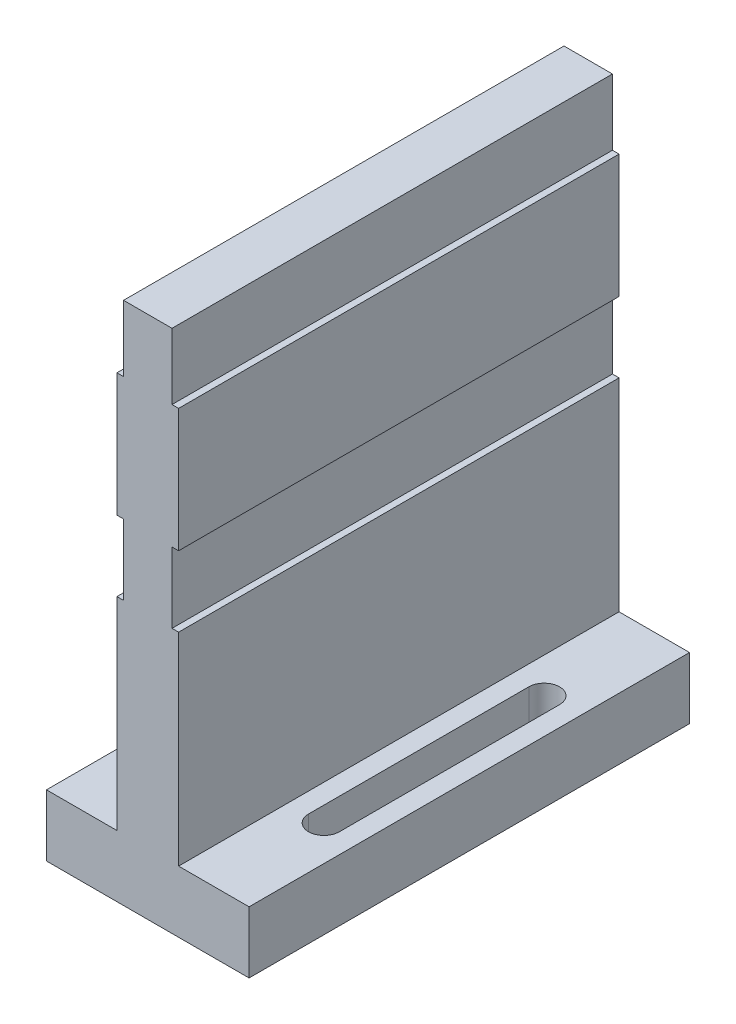
from build123d import *

# Parameters (mm, degrees)
EXTRUDE_1_DEPTH     = 50
CUT_EXTRUDE_1_REACH = 120.55
SKETCH_3_W          = 100
SKETCH_3_H          = 15
SKETCH_3_H_2        = 16
CUT_EXTRUDE_2_DEPTH = 1.5


with BuildPart() as part:
    # 草图1 → 凸台-拉伸1 (new, symmetric)
    with BuildSketch(Plane.XY):
        Polygon((0, 0), (23, 0), (23, 14), (7, 14), (7, 119), (-7, 119), (-7, 14), (-23, 14), (-23, 0), align=None)
    extrude(amount=EXTRUDE_1_DEPTH, both=True)

    # 草图2 → 切除-拉伸1 (cut, up to next)
    with BuildSketch(Plane(origin=(0, 14, 0), x_dir=(1, 0, 0), z_dir=(0, 1, 0)), mode=Mode.PRIVATE) as cut_extrude_1_sk1:
        with BuildLine():
            Line((11.5, -25), (11.5, 25))
            ThreePointArc((11.5, 25), (15, 28.5), (18.5, 25))
            Line((18.5, 25), (18.5, -25))
            ThreePointArc((18.5, -25), (15, -28.5), (11.5, -25))
        make_face()
    cut_extrude_1_tool1 = extrude(cut_extrude_1_sk1.sketch, amount=-CUT_EXTRUDE_1_REACH, mode=Mode.PRIVATE) & part.part
    cut_extrude_1 = cut_extrude_1_tool1.solids().sort_by_distance((15, 14, 0))[0]
    add(cut_extrude_1, mode=Mode.SUBTRACT)

    # 草图3 → 切除-拉伸2 (cut)
    with BuildSketch(Plane(origin=(7, 0, 0), x_dir=(0, 0, -1), z_dir=(1, 0, 0))):
        with Locations((0, 111.5)):
            Rectangle(SKETCH_3_W, SKETCH_3_H)
        with Locations((0, 68)):
            Rectangle(SKETCH_3_W, SKETCH_3_H_2)
    cut_extrude_2 = extrude(amount=-CUT_EXTRUDE_2_DEPTH, mode=Mode.SUBTRACT)

    # 镜向1: 切除-拉伸1 across plane
    add(cut_extrude_1.mirror(Plane(origin=(0, 0, 0), x_dir=(0, 0, 1), z_dir=(1, 0, 0))), mode=Mode.SUBTRACT)

    # 镜向2: 切除-拉伸2 across plane
    add(cut_extrude_2.mirror(Plane(origin=(0, 0, 0), x_dir=(0, 0, 1), z_dir=(1, 0, 0))), mode=Mode.SUBTRACT)


solid = part.part
